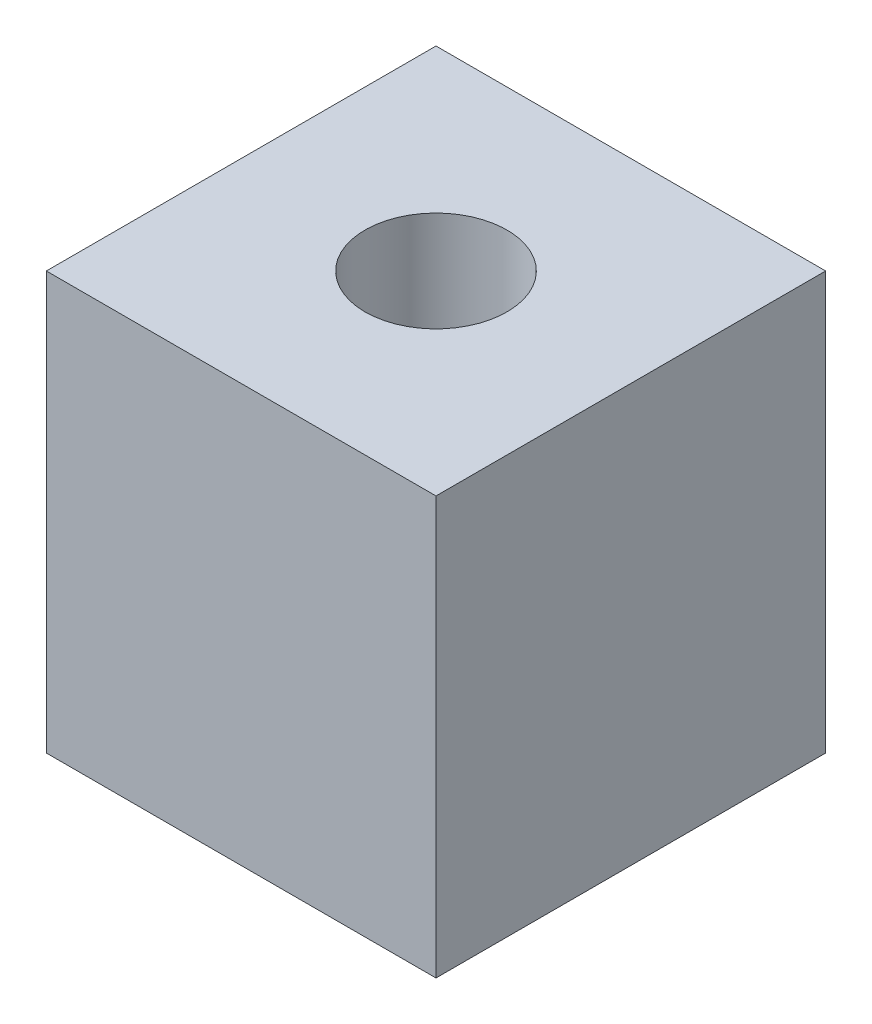
SolidWorks part; units mm, degrees
material "SS400B"
ref_plane "Front Plane" through (0, 0, 0) normal (0, 0, 1) x (1, 0, 0)
ref_plane "Top Plane" through (0, 0, 0) normal (0, 1, 0) x (1, 0, 0)
ref_plane "Right Plane" through (0, 0, 0) normal (1, 0, 0) x (0, 0, -1)
sketch "Sketch1" plane through (0, 0, 0) normal (0, 1, 0) x (1, 0, 0)
  line L1 (-14, 14) -> (14, 14)
  line L2 (-14, 14) -> (-14, -14)
  line L3 (-14, -14) -> (14, -14)
  line L4 (14, 14) -> (14, -14)
  line L5 (-14, 14) -> (14, -14) construction
  line L6 (-14, -14) -> (14, 14) construction
  circle A0 centre (0, 0) radius 5
  point P0 (0, 0)
  dimension "D3" = 10
  dimension "D1" = 28
  dimension "D2" = 28
extrude "Boss-Extrude1" add sketch "Sketch1" along normal blind 30
hole_wizard "M12 Tapped Hole1" positions "Sketch3" profile "Sketch4" tap size "M12" standard "GB" end condition through all
sketch "Sketch3" plane through (0, 30, 0) normal (0, 1, 0) x (1, 0, 0)
  point P0 (0, 0)
sketch "Sketch4" plane through (0, 30, 0) normal (1, 0, 0) x (0, 0, 1)
  line L0 (0, 0) -> (0, 30)
  line L1 (0, 30) -> (5.1, 30)
  line L2 (5.1, 30) -> (5.1, 0)
  line L5 (5.1, 0) -> (0, 0)
  line L11 (0, -6.35) -> (0, 107.95) construction
  dimension "通孔螺纹孔钻头直径" = 10.2
  dimension "通孔螺纹孔钻头深度" = 30
cosmetic thread "CosmeticThread1" parameters "D2"=12
